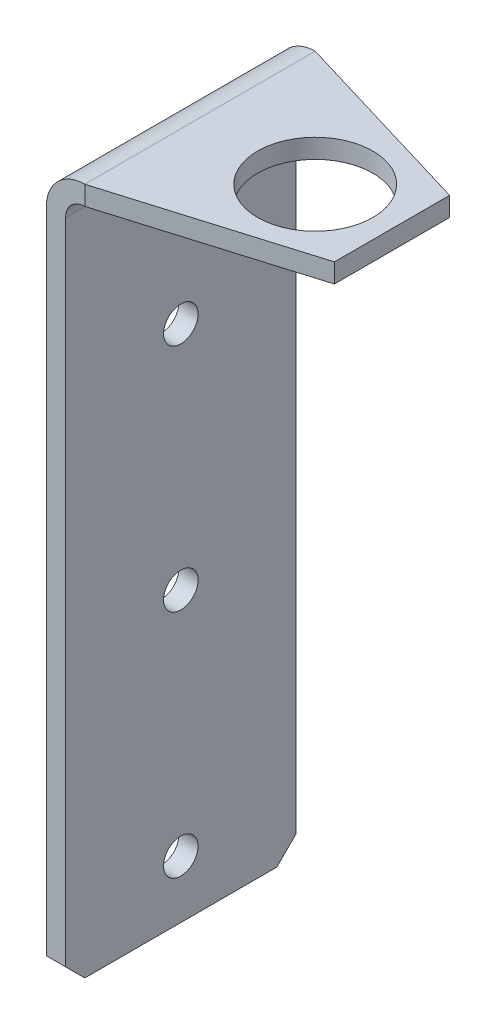
from build123d import *

# Parameters (mm, degrees)
BOSS_EXTRUDE1_DEPTH = 60
CHAMFER1_SIZE       = 5
SKETCH5_R           = 15
CUT_EXTRUDE1_DEPTH  = 60
CUT_EXTRUDE2_DEPTH  = 60
SKETCH3_R           = 4.5
CUT_EXTRUDE3_DEPTH  = 10


with BuildPart() as part:
    # Sketch1 → Boss-Extrude1 (new body)
    with BuildSketch(Plane.XY):
        with BuildLine():
            Line((0, 0), (0, 174))
            ThreePointArc((0, 174), (2.928932188, 181.071067812), (10, 184))
            Line((10, 184), (60, 184))
            Line((60, 184), (60, 179))
            Line((60, 179), (10, 179))
            ThreePointArc((10, 179), (6.464466094, 177.535533906), (5, 174))
            Line((5, 174), (5, 0))
            Line((5, 0), (0, 0))
        make_face()
    extrude(amount=BOSS_EXTRUDE1_DEPTH)

    # Chamfer1
    chamfer1_edges = [part.edges().sort_by_distance(p)[0] for p in [
        (2.5, 0, 0),
        (2.5, 0, 60),
    ]]
    chamfer(chamfer1_edges, length=CHAMFER1_SIZE)

    # Sketch5 → Cut-Extrude1 (cut)
    with BuildSketch(Plane(origin=(0, 184, 0), x_dir=(1, 0, 0), z_dir=(0, 1, 0))):
        with Locations(Location((40, -30, 0), (0, 0, 270))):
            Circle(SKETCH5_R)
    extrude(amount=-CUT_EXTRUDE1_DEPTH, mode=Mode.SUBTRACT)

    # Sketch6 → Cut-Extrude2 (cut)
    with BuildSketch(Plane(origin=(0, 184, 0), x_dir=(1, 0, 0), z_dir=(0, 1, 0))):
        Polygon((10, 0), (60, -15), (60, 0), align=None)
        Polygon((60, -45), (10, -60), (60, -60), align=None)
    extrude(amount=-CUT_EXTRUDE2_DEPTH, mode=Mode.SUBTRACT)

    # Sketch3 → Cut-Extrude3 (cut)
    with BuildSketch(Plane(origin=(5, 0, 0), x_dir=(0, 0, -1), z_dir=(1, 0, 0))):
        with Locations((-30, 15)):
            Circle(SKETCH3_R)
        with Locations((-30, 75)):
            Circle(SKETCH3_R)
        with Locations((-30, 135)):
            Circle(SKETCH3_R)
    extrude(amount=-CUT_EXTRUDE3_DEPTH, mode=Mode.SUBTRACT)


solid = part.part
